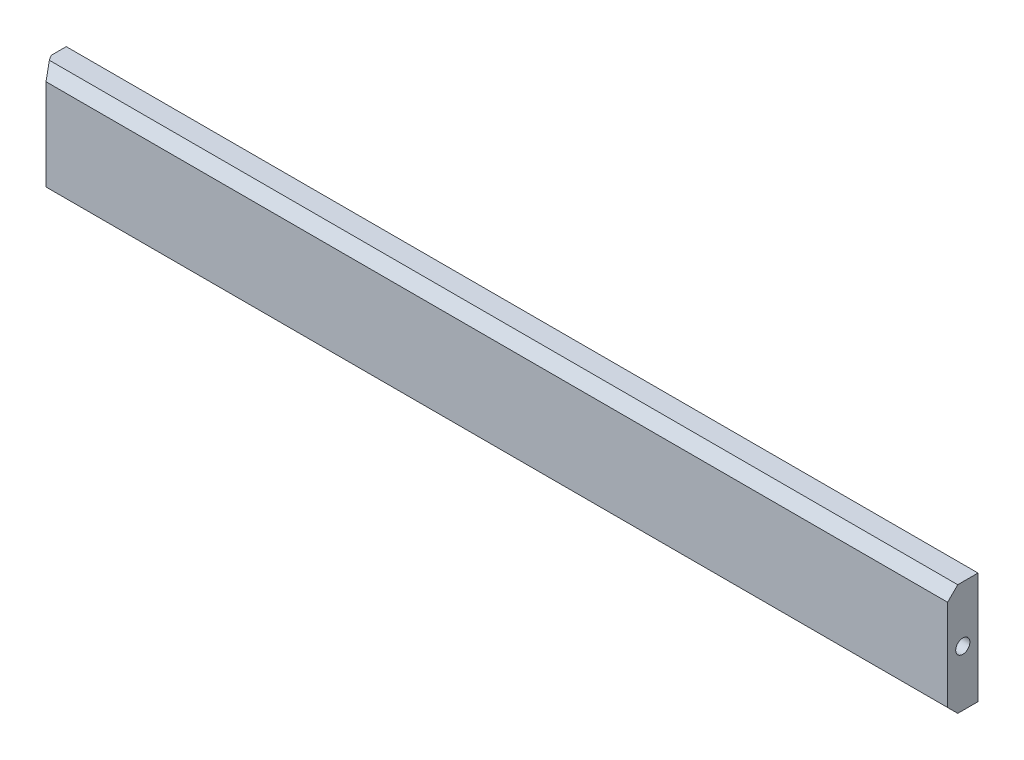
from build123d import *

# Parameters (mm, degrees)
SKETCH1_W              = 900
SKETCH1_H              = 110
BOSS_EXTRUDE1_DEPTH    = 30
CHAMFER1_SIZE          = 10
CHAMFER2_SIZE          = 15
CHAMFER2_SIZE2         = 10
M16_TAPPED_HOLE1_D     = 14
M16_TAPPED_HOLE1_DEPTH = 45
M16_TAPPED_HOLE1_TIP   = 4.206024333


with BuildPart() as part:
    # Sketch1 → Boss-Extrude1 (new body)
    with BuildSketch(Plane.XY):
        with Locations((450, 55)):
            Rectangle(SKETCH1_W, SKETCH1_H)
    extrude(amount=BOSS_EXTRUDE1_DEPTH)

    # Chamfer1
    chamfer1_edges = [part.edges().sort_by_distance(p)[0] for p in [
        (450, 110, 30),
        (450, 0, 30),
    ]]
    chamfer(chamfer1_edges, length=CHAMFER1_SIZE)

    # Chamfer2
    chamfer2_edges = [part.edges().sort_by_distance(p)[0] for p in [
        (0, 55, 30),
    ]]
    chamfer2_side = [part.faces().sort_by_distance(p)[0] for p in [
        (0, 55, 14.635416667),
    ]]
    chamfer(chamfer2_edges, length=CHAMFER2_SIZE, length2=CHAMFER2_SIZE2, reference=chamfer2_side[0])

    # M16 Tapped Hole1
    with Locations(Plane(origin=(900, 55, 15), x_dir=(0, 0, 1), z_dir=(1, 0, 0))):
        with Locations((0, 0)):
            Hole(M16_TAPPED_HOLE1_D / 2, depth=M16_TAPPED_HOLE1_DEPTH)
            with Locations((0, 0, -(M16_TAPPED_HOLE1_DEPTH + M16_TAPPED_HOLE1_TIP / 2))):  # 118° drill point
                Cone(0, M16_TAPPED_HOLE1_D / 2, M16_TAPPED_HOLE1_TIP, mode=Mode.SUBTRACT)


solid = part.part
